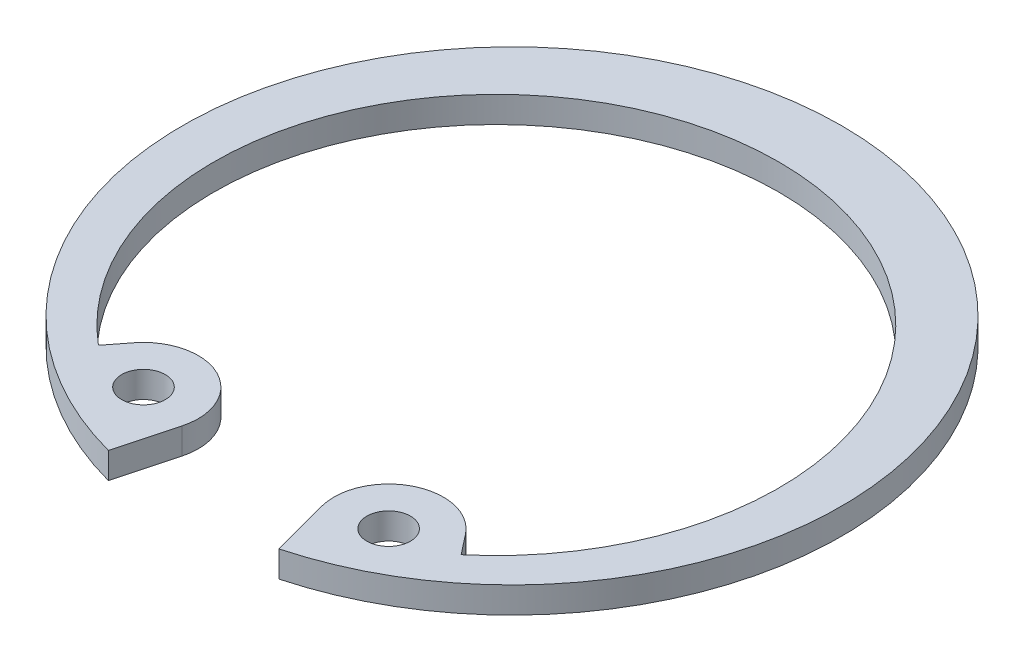
SolidWorks part; units mm, degrees
ref_plane "Front Plane" through (0, 0, 0) normal (0, 0, 1) x (1, 0, 0)
ref_plane "Top Plane" through (0, 0, 0) normal (0, 1, 0) x (1, 0, 0)
ref_plane "Right Plane" through (0, 0, 0) normal (1, 0, 0) x (0, 0, -1)
sketch "Sketch1" plane through (0, 0, 0) normal (0, 0, 1) x (1, 0, 0)
  line L1 (0, 0) -> (37.8, 0)
  line L2 (0, 0) -> (0, 1.5)
  line L3 (0, 1.5) -> (37.8, 1.5)
  line L4 (37.8, 0) -> (37.8, 1.5)
  line L5 (0, 0) -> (3.6, 0)
  line L6 (0, 0) -> (0, 2.5)
  line L7 (0, 2.5) -> (3.6, 2.5)
  line L8 (3.6, 0) -> (3.6, 2.5)
  dimension "D3" = 37.8
  dimension "T" = 1.5
  dimension "C" = 3.6
  dimension "D0" = 2.5
sketch "Sketch2" plane through (0, 0, 0) normal (0, 1, 0) x (1, 0, 0)
  line L0 (0, 18.9) -> (0, 15.3) construction
  line L1 (-10.4011, -13.32) -> (-9.5051, -12.1726)
  line L2 (-3.9972, -14.9178) -> (-4.8917, -18.256)
  line L3 (0, 1.6194) -> (0, -3.957) construction
  line L4 (3.9972, -14.9178) -> (4.8917, -18.256)
  line L5 (0, 0) -> (-7.0302, -14.1051) construction
  line L6 (10.4011, -13.32) -> (9.5051, -12.1726)
  arc A0 (4.8917, -18.256) -> (-4.8917, -18.256) centre (0, 0) ccw
  arc A2 (-3.9972, -14.9178) -> (-9.5051, -12.1726) centre (-7.0302, -14.1051) ccw
  circle A3 centre (-7.0302, -14.1051) radius 1.25
  circle A4 centre (7.0302, -14.1051) radius 1.25
  arc A5 (3.9972, -14.9178) -> (9.5051, -12.1726) centre (7.0302, -14.1051) cw
  arc A7 (10.4011, -13.32) -> (-10.4011, -13.32) centre (0, -0.9) ccw
  dimension "D1" = 37.8
  dimension "D3" = 32.4
  dimension "D5" = 2.5
  dimension "D6" = 6.28
  dimension "D2" = 3.6
  dimension "D4" = 15
  dimension "D7" = 15.76
extrude "Boss-Extrude1" add sketch "Sketch2" along normal blind 1.5
